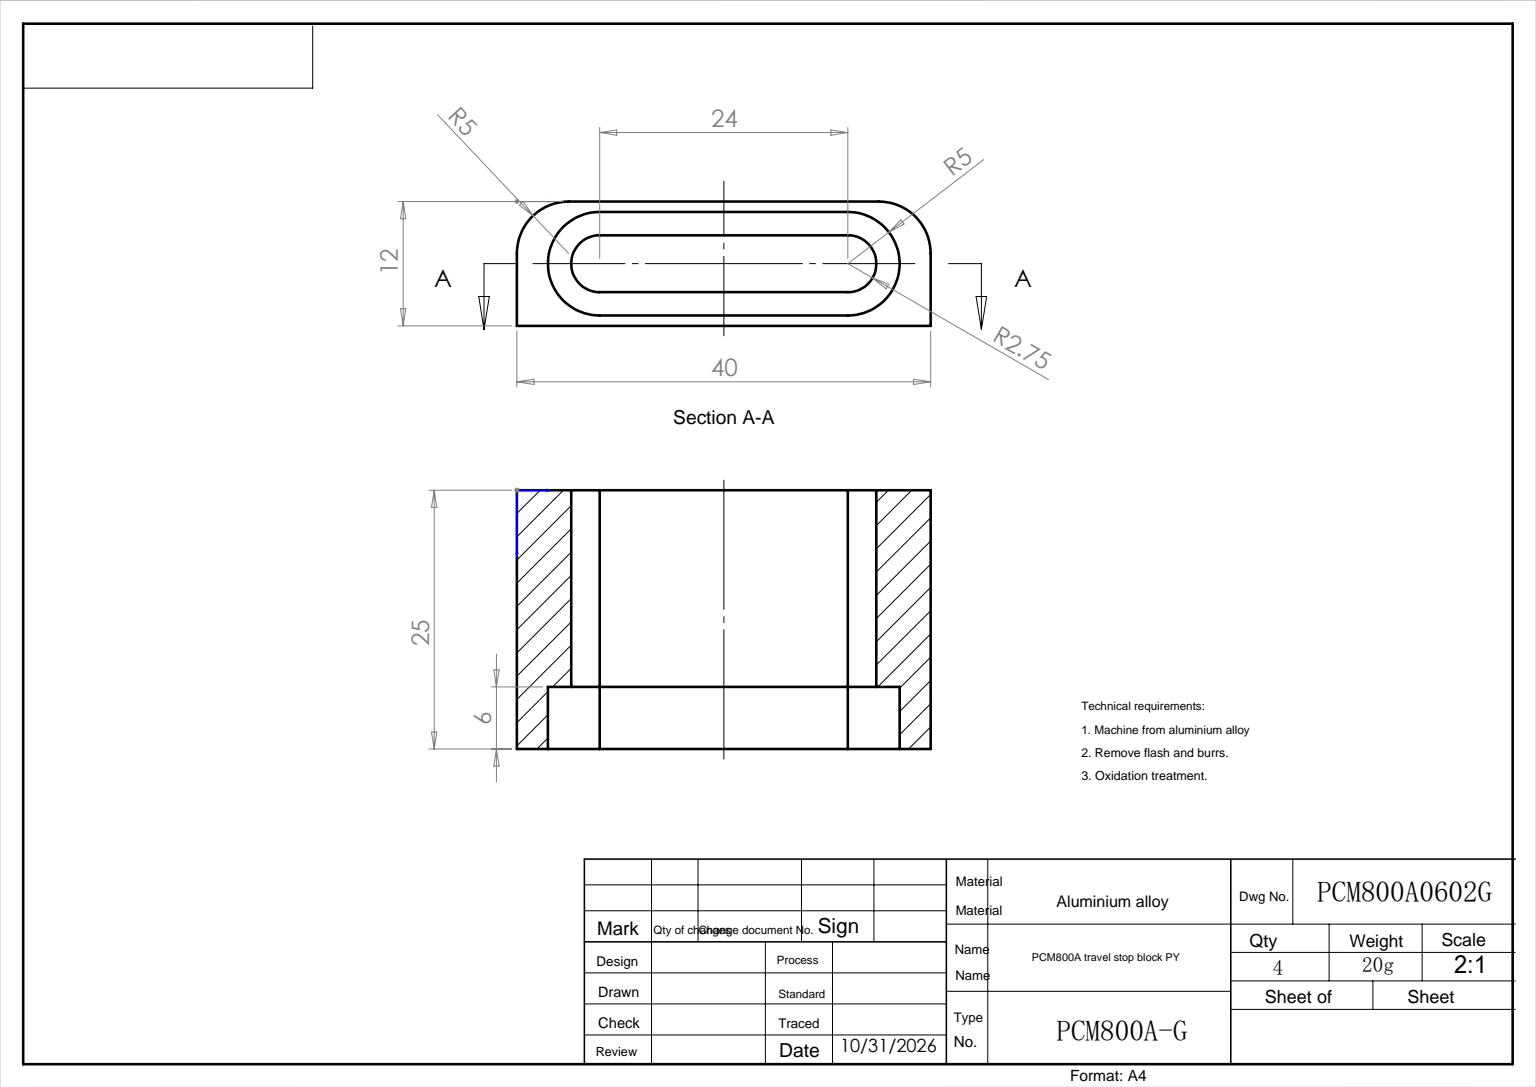
SolidWorks part; units mm, degrees
ref_plane "前视基准面" through (0, 0, 0) normal (0, 0, 1) x (1, 0, 0)
ref_plane "上视基准面" through (0, 0, 0) normal (0, 1, 0) x (1, 0, 0)
ref_plane "右视基准面" through (0, 0, 0) normal (1, 0, 0) x (0, 0, -1)
sketch "草图1" plane through (0, 0, 0) normal (0, 0, 1) x (1, 0, 0)
  line L1 (0, 0) -> (40, 0)
  line L2 (0, 0) -> (0, 25)
  line L3 (0, 25) -> (40, 25)
  line L4 (40, 0) -> (40, 25)
  dimension "D1" = 25
  dimension "D2" = 40
extrude "凸台-拉伸1" add sketch "草图1" along normal blind 12
sketch "草图4" plane through (0, 25, 0) normal (0, 1, 0) x (1, 0, 0)
  line L0 (0, -6) -> (42.7149, -6) construction
  line L1 (0, -12) -> (0, 0) construction
  line L2 (8, -1) -> (32, -1)
  line L3 (8, -11) -> (32, -11)
  line L4 (20, 0) -> (20, -17.202) construction
  line L5 (40, 0) -> (0, 0) construction
  arc A0 (8, -1) -> (8, -11) centre (8, -6) ccw
  arc A1 (32, -11) -> (32, -1) centre (32, -6) ccw
  dimension "D1" = 5
  dimension "D2" = 12
  dimension "D3" = 12
extrude "切除-拉伸1" cut sketch "草图4" against normal blind 6
sketch "草图5" plane through (0, 19, 0) normal (0, 1, 0) x (1, 0, 0)
  line L8 (8, -8.75) -> (32, -8.75)
  line L9 (32, -3.25) -> (8, -3.25)
  line L10 (8, -8.75) -> (32, -8.75)
  line L11 (32, -3.25) -> (8, -3.25)
  arc A12 (32, -8.75) -> (32, -3.25) centre (32, -6) ccw
  arc A13 (8, -3.25) -> (8, -8.75) centre (8, -6) ccw
  arc A14 (32, -8.75) -> (32, -3.25) centre (32, -6) ccw
  arc A15 (8, -3.25) -> (8, -8.75) centre (8, -6) ccw
  dimension "D1" = 2.25
extrude "切除-拉伸2" cut sketch "草图5" against normal blind 19
fillet "圆角1" radius 5 2 edges at (0, 12.5, 0) (40, 12.5, 0)
